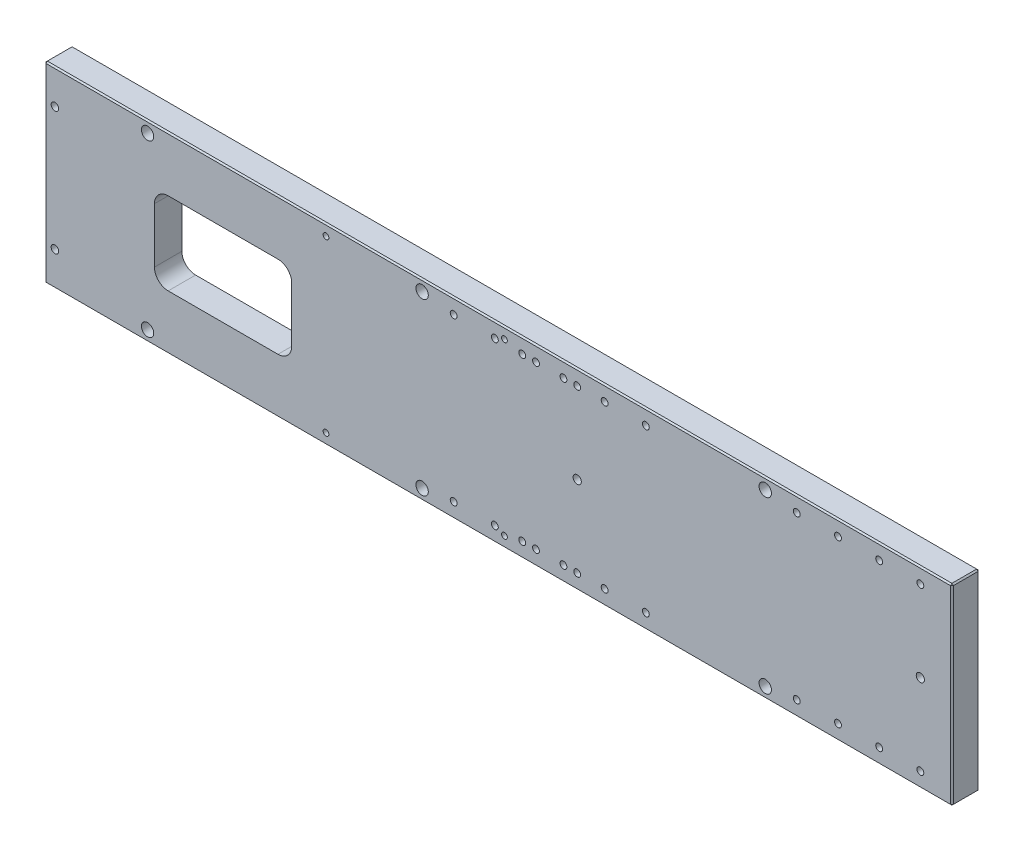
from build123d import *

# Parameters (mm, degrees)
SKETCH_1_W               = 661
SKETCH_1_H               = 140
EXTRUDE_1_DEPTH          = 20
CHAMFER_1_SIZE           = 1
HOLE_WIZARD_M5_1_D       = 4.2
HOLE_WIZARD_M6_1_D       = 5
SKETCH_18_R              = 3
CUT_EXTRUDE_4_DEPTH      = 339.42318183
HOLE_WIZARD_1_AT_2_COUNT = 2
HOLE_WIZARD_1_AT_2_PITCH = 90
HOLE1_D                  = 9
HOLE1_CBORE_D            = 15
HOLE1_CBORE_DEPTH        = 8.5
SKETCH_21_W              = 100
SKETCH_21_H              = 60
CUT_EXTRUDE_5_DEPTH      = 339.42318183
FILLET_2_R               = 10


with BuildPart() as part:
    # 草图1 → 凸台-拉伸1 (new body)
    with BuildSketch(Plane.XY):
        Rectangle(SKETCH_1_W, SKETCH_1_H)
    extrude(amount=EXTRUDE_1_DEPTH)

    # 倒角1
    chamfer_1_edges = [part.edges().sort_by_distance(p)[0] for p in [
        (-330.5, 0, 20),
        (0, -70, 20),
        (330.5, 0, 20),
        (0, -70, 0),
        (-330.5, 0, 0),
        (0, 70, 0),
        (330.5, 0, 0),
        (0, 70, 20),
        (330.5, -70, 10),
        (-330.5, -70, 10),
        (-330.5, 70, 10),
        (330.5, 70, 10),
    ]]
    chamfer(chamfer_1_edges, length=CHAMFER_1_SIZE)

    # M5 螺纹孔1 (through all)
    with Locations(Plane.XY.offset(20)):
        with Locations((4.5, 62), (4.5, -62), (-125.5, 62), (-125.5, -62), (-255.5, -62), (-255.5, 62)):
            Hole(HOLE_WIZARD_M5_1_D / 2)

    # M6 螺纹孔1 (through all)
    with Locations(Plane.XY.offset(20)):
        with Locations((307.5, -58.999999026), (107.5, -58.999999026), (57.5, -58.999999026), (57.5, 59.000000974), (107.5, 59.000000974), (307.5, 59.000000974), (277.5, -58.999999026), (77.5, -58.999999026), (27.5, -58.999999026), (27.5, 59.000000974), (77.5, 59.000000974), (277.5, 59.000000974), (247.5, -58.999999026), (47.5, -58.999999026), (-2.5, -58.999999026), (-2.5, 59.000000974), (47.5, 59.000000974), (247.5, 59.000000974), (217.5, -58.999999026), (17.5, -58.999999026), (-32.5, -58.999999026), (-32.5, 59.000000974), (17.5, 59.000000974), (217.5, 59.000000974)):
            Hole(HOLE_WIZARD_M6_1_D / 2)

    # 草图18 → 切除-拉伸4 (cut, through all)
    with BuildSketch(Plane.XY.offset(20)):
        with Locations((307.5, 9.74e-07)):
            Circle(SKETCH_18_R)
        with Locations((57.5, 9.74e-07)):
            Circle(SKETCH_18_R)
    extrude(amount=-CUT_EXTRUDE_4_DEPTH, mode=Mode.SUBTRACT)

    # 草图20 → 打孔尺寸(%根据)内六角圆柱头螺钉的类型1 (revolve, cut)
    with BuildSketch(Plane(origin=(-323, 45, 0), x_dir=(0, 1, 0), z_dir=(1, 0, 0))):
        Polygon((0, 0), (0, 20), (2.75, 20), (2.75, 5.7), (5, 5.7), (5, 0.525), (5.525, 0), align=None)
    hole_wizard_1 = revolve(axis=Axis((-323, 45, -6.35), (0, 0, 1)), mode=Mode.SUBTRACT)

    # 打孔尺寸(%根据)内六角圆柱头螺钉的类型1 at 2: 打孔尺寸(%根据)内六角圆柱头螺钉的类型1 ×2
    with Locations(*[(0, -i * HOLE_WIZARD_1_AT_2_PITCH, 0) for i in range(1, HOLE_WIZARD_1_AT_2_COUNT)]):
        add(hole_wizard_1, mode=Mode.SUBTRACT)

    # Hole1 (through all)
    with Locations(Plane(origin=(-242.630892878, -61.065000019, 0), x_dir=(-1, 0, 0), z_dir=(0, 0, -1))):
        with Locations((12.869107122, -0.934999981), (-187.130892878, -0.934999981), (-437.130892878, -0.934999981), (-437.130892878, 123.065000019), (-187.130892878, 123.065000019), (12.869107122, 123.065000019)):
            CounterBoreHole(HOLE1_D / 2, HOLE1_CBORE_D / 2, HOLE1_CBORE_DEPTH)

    # 草图21 → 切除-拉伸5 (cut, through all)
    with BuildSketch(Plane(origin=(0, 0, 0), x_dir=(-1, 0, 0), z_dir=(0, 0, -1))):
        with Locations((200.5, 0)):
            Rectangle(SKETCH_21_W, SKETCH_21_H)
    extrude(amount=-CUT_EXTRUDE_5_DEPTH, mode=Mode.SUBTRACT)

    # 圆角2
    fillet_2_edges = [part.edges().sort_by_distance(p)[0] for p in [
        (-150.5, -30, 10),
        (-150.5, 30, 10),
        (-250.5, 30, 10),
        (-250.5, -30, 10),
    ]]
    fillet(fillet_2_edges, radius=FILLET_2_R)


solid = part.part
